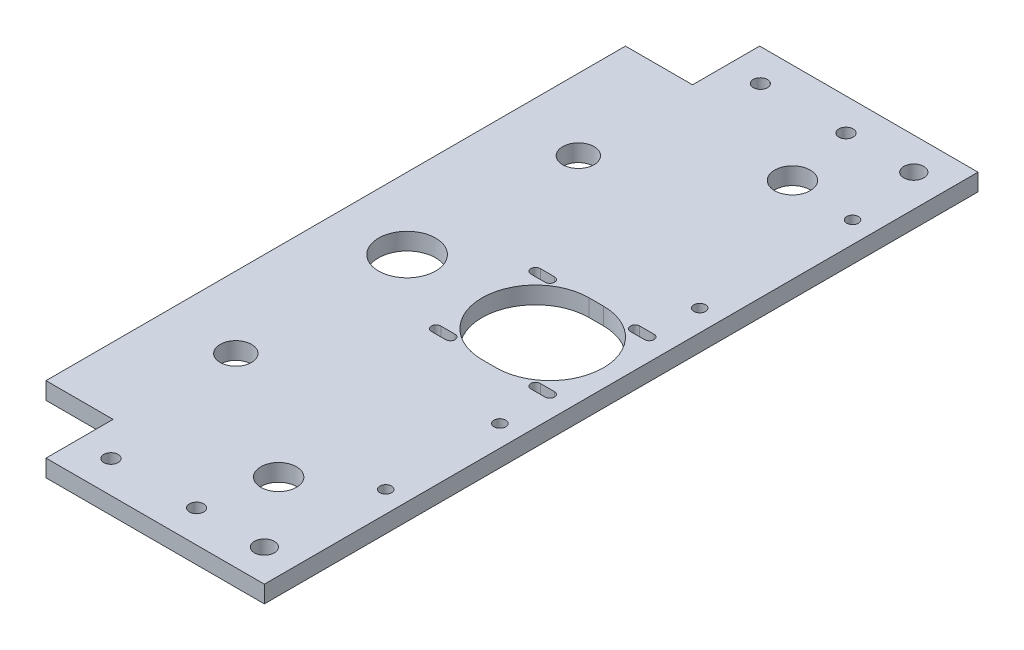
from build123d import *

# Parameters (mm, degrees)
SKETCH1_W                      = 200
SKETCH1_H                      = 500
BOSS_EXTRUDE1_DEPTH            = 12
SKETCH2_R                      = 20
SKETCH2_R_2                    = 11
CUT_EXTRUDE1_DEPTH             = 12
SKETCH4_R                      = 12.5
CUT_EXTRUDE3_DEPTH             = 12
SKETCH5_R                      = 7
CUT_EXTRUDE4_DEPTH             = 12
F_8_2_8_2_DIAMETER_HOLE1_D     = 8.2
F_8_2_8_2_DIAMETER_HOLE1_DEPTH = 13
F_8_2_8_2_DIAMETER_HOLE1_TIP   = 2.463528538
F_10_0_10_DIAMETER_HOLE1_D     = 10
SKETCH11_W                     = 47
SKETCH11_H                     = 47
CUT_EXTRUDE6_DEPTH             = 270.525508997
CUT_EXTRUDE7_DEPTH             = 270.525508997
F_5_0_5_DIAMETER_HOLE1_D       = 5
CUT_EXTRUDE8_DEPTH             = 270.525508997


with BuildPart() as part:
    # Sketch1 → Boss-Extrude1 (new body)
    with BuildSketch(Plane(origin=(0, 0, 0), x_dir=(1, 0, 0), z_dir=(0, 1, 0))):
        Rectangle(SKETCH1_W, SKETCH1_H)
    extrude(amount=BOSS_EXTRUDE1_DEPTH)

    # Sketch2 → Cut-Extrude1 (cut)
    with BuildSketch(Plane(origin=(0, 12, 0), x_dir=(1, 0, 0), z_dir=(0, 1, 0))):
        with Locations(Location((-50, 0, 0), (0, 0, 270))):
            Circle(SKETCH2_R)
        with Locations(Location((-50, 120, 0), (0, 0, 270))):
            Circle(SKETCH2_R_2)
        with Locations(Location((-50, -120, 0), (0, 0, 90))):
            Circle(SKETCH2_R_2)
    extrude(amount=-CUT_EXTRUDE1_DEPTH, mode=Mode.SUBTRACT)

    # Sketch4 → Cut-Extrude3 (cut)
    with BuildSketch(Plane(origin=(0, 12, 0), x_dir=(1, 0, 0), z_dir=(0, 1, 0))):
        with Locations(Location((40, 180, 0), (0, 0, 270))):
            Circle(SKETCH4_R)
        with Locations(Location((40, -180, 0), (0, 0, 90))):
            Circle(SKETCH4_R)
    extrude(amount=-CUT_EXTRUDE3_DEPTH, mode=Mode.SUBTRACT)

    # Sketch5 → Cut-Extrude4 (cut)
    with BuildSketch(Plane(origin=(0, 12, 0), x_dir=(1, 0, 0), z_dir=(0, 1, 0))):
        with Locations(Location((-77.5, 227.5, 0), (0, 0, 270))):
            Circle(SKETCH5_R)
        with Locations(Location((77.5, 227.5, 0), (0, 0, 270))):
            Circle(SKETCH5_R)
        with Locations(Location((-77.5, -227.5, 0), (0, 0, 270))):
            Circle(SKETCH5_R)
        with Locations(Location((77.5, -227.5, 0), (0, 0, 270))):
            Circle(SKETCH5_R)
    extrude(amount=-CUT_EXTRUDE4_DEPTH, mode=Mode.SUBTRACT)

    # Ø8.2 (8.2) Diameter Hole1
    with Locations(Plane(origin=(0, 12, 0), x_dir=(1, 0, 0), z_dir=(0, 1, 0))):
        with Locations((85, 177.098099642), (85, 70), (85, -70), (85, -150)):
            Hole(F_8_2_8_2_DIAMETER_HOLE1_D / 2, depth=F_8_2_8_2_DIAMETER_HOLE1_DEPTH)
            with Locations((0, 0, -(F_8_2_8_2_DIAMETER_HOLE1_DEPTH + F_8_2_8_2_DIAMETER_HOLE1_TIP / 2))):  # 118° drill point
                Cone(0, F_8_2_8_2_DIAMETER_HOLE1_D / 2, F_8_2_8_2_DIAMETER_HOLE1_TIP, mode=Mode.SUBTRACT)

    # Ø10.0 (10) Diameter Hole1 (through all)
    with Locations(Plane(origin=(0, 12, 0), x_dir=(1, 0, 0), z_dir=(0, 1, 0))):
        with Locations((-30, 227.5), (30, 227.5), (30, -227.5), (-30, -227.5)):
            Hole(F_10_0_10_DIAMETER_HOLE1_D / 2)

    # Sketch11 → Cut-Extrude6 (cut, through all)
    with BuildSketch(Plane(origin=(0, 12, 0), x_dir=(1, 0, 0), z_dir=(0, 1, 0))):
        with Locations((-76.5, 226.5)):
            Rectangle(SKETCH11_W, SKETCH11_H)
        with Locations((-76.5, -226.5)):
            Rectangle(SKETCH11_W, SKETCH11_H)
    extrude(amount=-CUT_EXTRUDE6_DEPTH, mode=Mode.SUBTRACT)

    # Sketch3 → Cut-Extrude7 (cut, through all)
    with BuildSketch(Plane(origin=(0, 12, 0), x_dir=(1, 0, 0), z_dir=(0, 1, 0))):
        with BuildLine():
            Line((50, -37.5), (40, -37.5))
            ThreePointArc((40, -37.5), (2.5, 0), (40, 37.5))
            Line((40, 37.5), (50, 37.5))
            ThreePointArc((50, 37.5), (87.5, 0), (50, -37.5))
        make_face()
    extrude(amount=-CUT_EXTRUDE7_DEPTH, mode=Mode.SUBTRACT)

    # Ø5.0 (5) Diameter Hole1 (through all)
    with Locations(Plane(origin=(0, 12, 0), x_dir=(1, 0, 0), z_dir=(0, 1, 0))):
        with Locations((5.15, 34.85), (5.15, -34.85), (74.85, -34.85), (74.85, 34.85)):
            Hole(F_5_0_5_DIAMETER_HOLE1_D / 2)

    # Sketch16 → Cut-Extrude8 (cut, through all)
    with BuildSketch(Plane(origin=(0, 12, 0), x_dir=(1, 0, 0), z_dir=(0, 1, 0))):
        with BuildLine():
            Line((5.15, 38.15), (15.15, 38.15))
            ThreePointArc((15.15, 38.15), (18.45, 34.85), (15.15, 31.55))
            Line((15.15, 31.55), (5.15, 31.55))
            ThreePointArc((5.15, 31.55), (1.85, 34.85), (5.15, 38.15))
        make_face()
        with BuildLine():
            Line((74.85, 38.15), (84.85, 38.15))
            ThreePointArc((84.85, 38.15), (88.15, 34.85), (84.85, 31.55))
            Line((84.85, 31.55), (74.85, 31.55))
            ThreePointArc((74.85, 31.55), (71.55, 34.85), (74.85, 38.15))
        make_face()
        with BuildLine():
            Line((5.15, -31.55), (15.15, -31.55))
            ThreePointArc((15.15, -31.55), (18.45, -34.85), (15.15, -38.15))
            Line((15.15, -38.15), (5.15, -38.15))
            ThreePointArc((5.15, -38.15), (1.85, -34.85), (5.15, -31.55))
        make_face()
        with BuildLine():
            Line((74.85, -31.55), (84.85, -31.55))
            ThreePointArc((84.85, -31.55), (88.15, -34.85), (84.85, -38.15))
            Line((84.85, -38.15), (74.85, -38.15))
            ThreePointArc((74.85, -38.15), (71.55, -34.85), (74.85, -31.55))
        make_face()
    extrude(amount=-CUT_EXTRUDE8_DEPTH, mode=Mode.SUBTRACT)


solid = part.part
